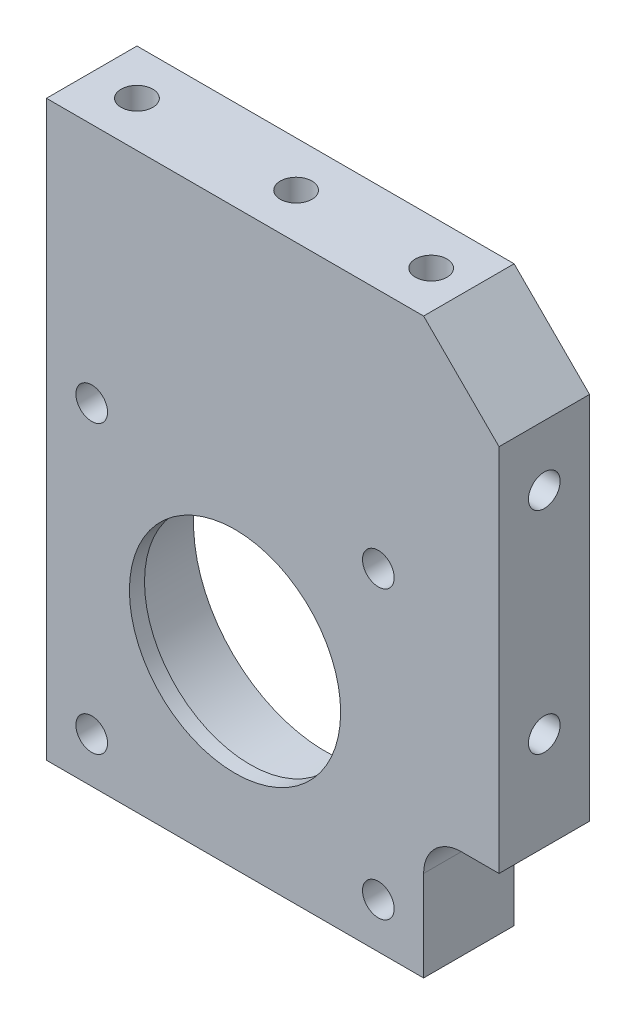
from build123d import *

# Parameters (mm, degrees)
SKETCH_1_W             = 60
SKETCH_1_H             = 82
EXTRUDE_1_DEPTH        = 6
SKETCH_10_R            = 17.5
CUT_EXTRUDE_1_DEPTH    = 10
SKETCH_12_R            = 14
CUT_EXTRUDE_2_DEPTH    = 52.778373864
SKETCH_13_W            = 10
SKETCH_13_H            = 22
CUT_EXTRUDE_3_DEPTH    = 53.201532545
FILLET_1_R             = 5
HOLE_WIZARD_M5_2_D     = 4.2
MOVE_FACE_1_BY         = 1
CHAMFER_2_SIZE         = 10
HOLE_WIZARD_M5_3_D     = 4.2
HOLE_WIZARD_M5_3_DEPTH = 12.4
HOLE_WIZARD_M5_3_TIP   = 1.2618073
HOLE_WIZARD_M5_4_D     = 4.2
HOLE_WIZARD_M5_4_DEPTH = 12.4
HOLE_WIZARD_M5_4_TIP   = 1.2618073
MOVE_FACE_3_BY         = 5


with BuildPart() as part:
    # 草图1 → 凸台-拉伸1 (new, symmetric)
    with BuildSketch(Plane.XY):
        Rectangle(SKETCH_1_W, SKETCH_1_H)
    extrude(amount=EXTRUDE_1_DEPTH, both=True)

    # 草图10 → 切除-拉伸1 (cut)
    with BuildSketch(Plane.XY.offset(-6)):
        with Locations((-5, -11)):
            Circle(SKETCH_10_R)
    extrude(amount=CUT_EXTRUDE_1_DEPTH, mode=Mode.SUBTRACT)

    # 草图12 → 切除-拉伸2 (cut, through all)
    with BuildSketch(Plane(origin=(0, 0, 4), x_dir=(-1, 0, 0), z_dir=(0, 0, -1))):
        with Locations((5, -11)):
            Circle(SKETCH_12_R)
    extrude(amount=-CUT_EXTRUDE_2_DEPTH, mode=Mode.SUBTRACT)

    # 草图13 → 切除-拉伸3 (cut, through all)
    with BuildSketch(Plane.XY.offset(6)):
        with Locations((25, -30)):
            Rectangle(SKETCH_13_W, SKETCH_13_H)
    extrude(amount=-CUT_EXTRUDE_3_DEPTH, mode=Mode.SUBTRACT)

    # 圆角1
    fillet_1_edges = [part.edges().sort_by_distance(p)[0] for p in [
        (20, -19, 0),
    ]]
    fillet(fillet_1_edges, radius=FILLET_1_R)

    # M5 螺纹孔2 (through all)
    with Locations(Plane(origin=(0, 0, -6), x_dir=(-1, 0, 0), z_dir=(0, 0, -1))):
        with Locations((-14, 8), (-14, -30), (24, -30), (24, 8)):
            Hole(HOLE_WIZARD_M5_2_D / 2)

    # Move Face 1: a face moved inward by 1.0
    extrude(part.faces().sort_by_distance((0, 41, 0))[0], amount=MOVE_FACE_1_BY, dir=(0, -1, 0), mode=Mode.SUBTRACT)

    # 倒角2
    chamfer_2_edges = [part.edges().sort_by_distance(p)[0] for p in [
        (30, 40, 0),
    ]]
    chamfer(chamfer_2_edges, length=CHAMFER_2_SIZE)

    # M5 螺纹孔3
    with Locations(Plane(origin=(0, 40, 0), x_dir=(1, 0, 0), z_dir=(0, 1, 0))):
        with Locations((-24, 0), (-2.9, 0), (15, 0)):
            Hole(HOLE_WIZARD_M5_3_D / 2, depth=HOLE_WIZARD_M5_3_DEPTH)
            with Locations((0, 0, -(HOLE_WIZARD_M5_3_DEPTH + HOLE_WIZARD_M5_3_TIP / 2))):  # 118° drill point
                Cone(0, HOLE_WIZARD_M5_3_D / 2, HOLE_WIZARD_M5_3_TIP, mode=Mode.SUBTRACT)

    # M5 螺纹孔4
    with Locations(Plane(origin=(30, 0, 0), x_dir=(0, 0, -1), z_dir=(1, 0, 0))):
        with Locations((0, 22), (0, -6)):
            Hole(HOLE_WIZARD_M5_4_D / 2, depth=HOLE_WIZARD_M5_4_DEPTH)
            with Locations((0, 0, -(HOLE_WIZARD_M5_4_DEPTH + HOLE_WIZARD_M5_4_TIP / 2))):  # 118° drill point
                Cone(0, HOLE_WIZARD_M5_4_D / 2, HOLE_WIZARD_M5_4_TIP, mode=Mode.SUBTRACT)

    # Move Face 3: a face moved inward by 5.0
    extrude(part.faces().sort_by_distance((-5, -41, 0))[0], amount=MOVE_FACE_3_BY, dir=(0, 1, 0), mode=Mode.SUBTRACT)


solid = part.part
